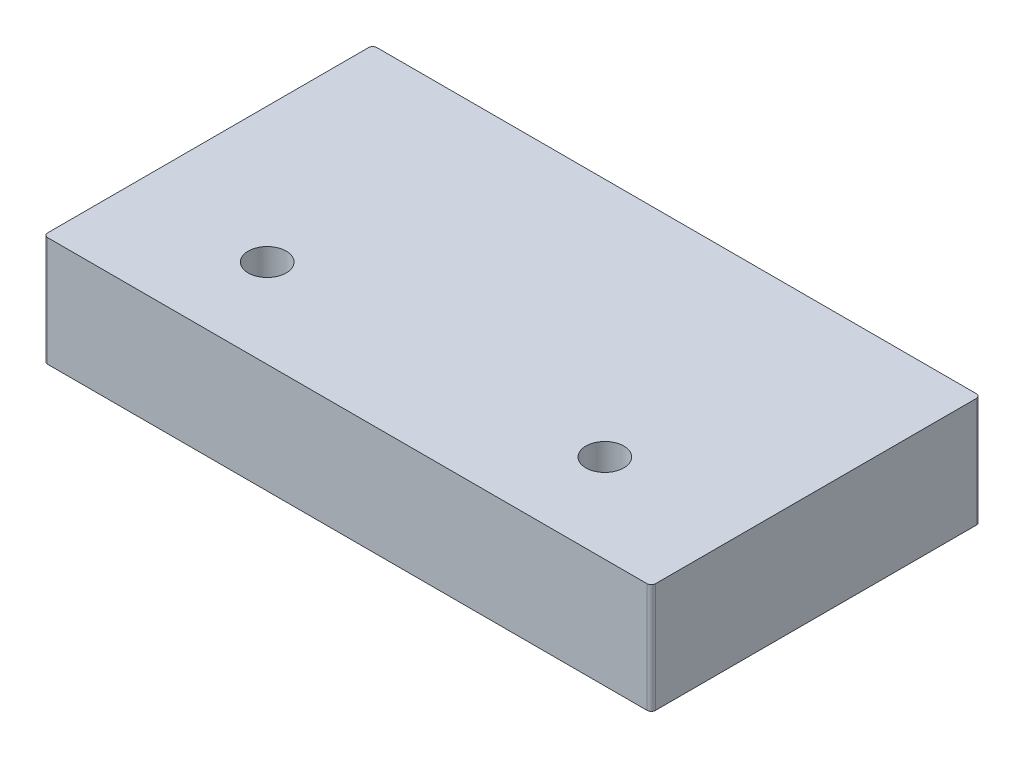
SolidWorks part; units mm, degrees
ref_plane "前视基准面" through (0, 0, 0) normal (0, 0, 1) x (1, 0, 0)
ref_plane "上视基准面" through (0, 0, 0) normal (0, 1, 0) x (1, 0, 0)
ref_plane "右视基准面" through (0, 0, 0) normal (1, 0, 0) x (0, 0, -1)
sketch "草图1" plane through (0, 0, 0) normal (0, 0, 1) x (1, 0, 0)
  line L1 (36, 6.5) -> (-36, 6.5)
  line L2 (36, 6.5) -> (36, -6.5)
  line L3 (36, -6.5) -> (-36, -6.5)
  line L4 (-36, 6.5) -> (-36, -6.5)
  line L5 (36, 6.5) -> (-36, -6.5) construction
  line L6 (36, -6.5) -> (-36, 6.5) construction
  point P0 (0, 0)
  dimension "D1" = 13
  dimension "D2" = 72
extrude "凸台-拉伸1" add sketch "草图1" along normal blind 39
fillet "圆角1" radius 0.5 4 edges at (36, 0, 0) (36, 0, 39) (-36, 0, 39) (-36, 0, 0)
sketch "草图2" plane through (0, 6.5, 0) normal (0, 1, 0) x (1, 0, 0)
  line L0 (-20, -28.5) -> (20, -28.5) construction
  line L1 (35.5, -39) -> (-35.5, -39) construction
  circle A0 centre (-20, -28.5) radius 2.25
  circle A1 centre (20, -28.5) radius 2.25
  point P4 (0, -28.5)
  dimension "D3" = 4.5
  dimension "D4" = 4.5
  dimension "D1" = 40
  dimension "D2" = 10.5
extrude "切除-拉伸1" cut sketch "草图2" against normal through all
